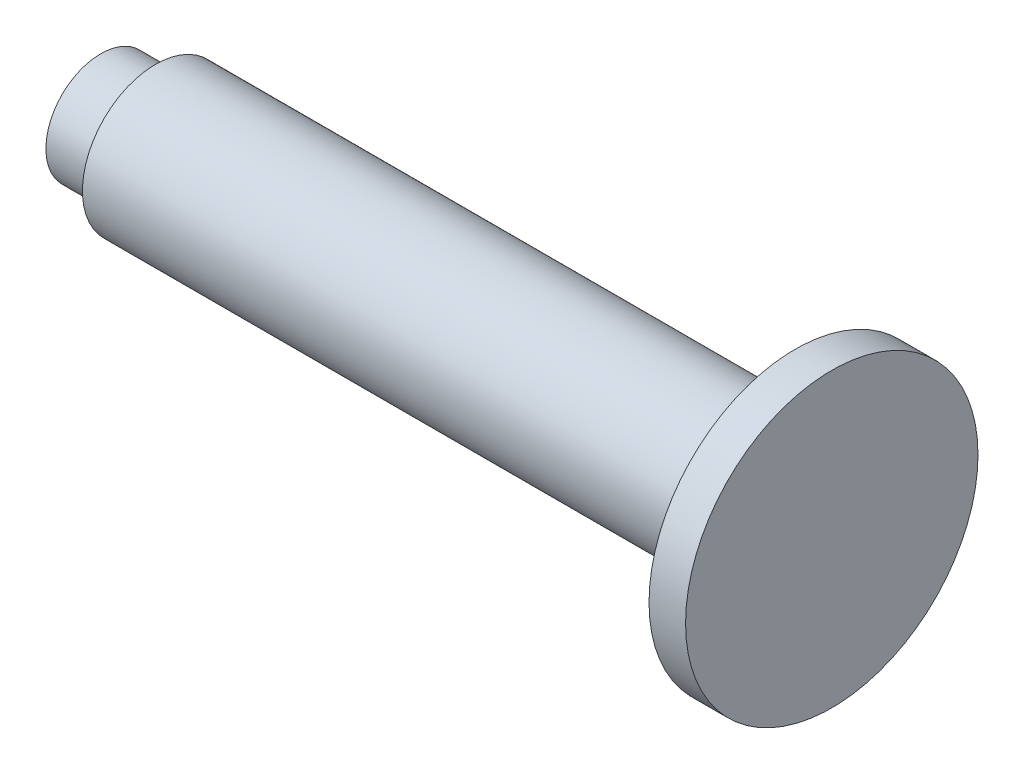
from build123d import *


with BuildPart() as part:
    # Sketch1 → Revolve1 (revolve)
    with BuildSketch(Plane.XY, mode=Mode.PRIVATE) as revolve1_sk:
        Polygon((0, 0), (0, 3), (3, 3), (3, 4), (38, 4), (38, 8), (40, 8), (40, 0), align=None)
    revolve(revolve1_sk.sketch.rotate(Axis((40, 0, 0), (-1, 0, 0)), 90), axis=Axis((40, 0, 0), (-1, 0, 0)))


solid = part.part
